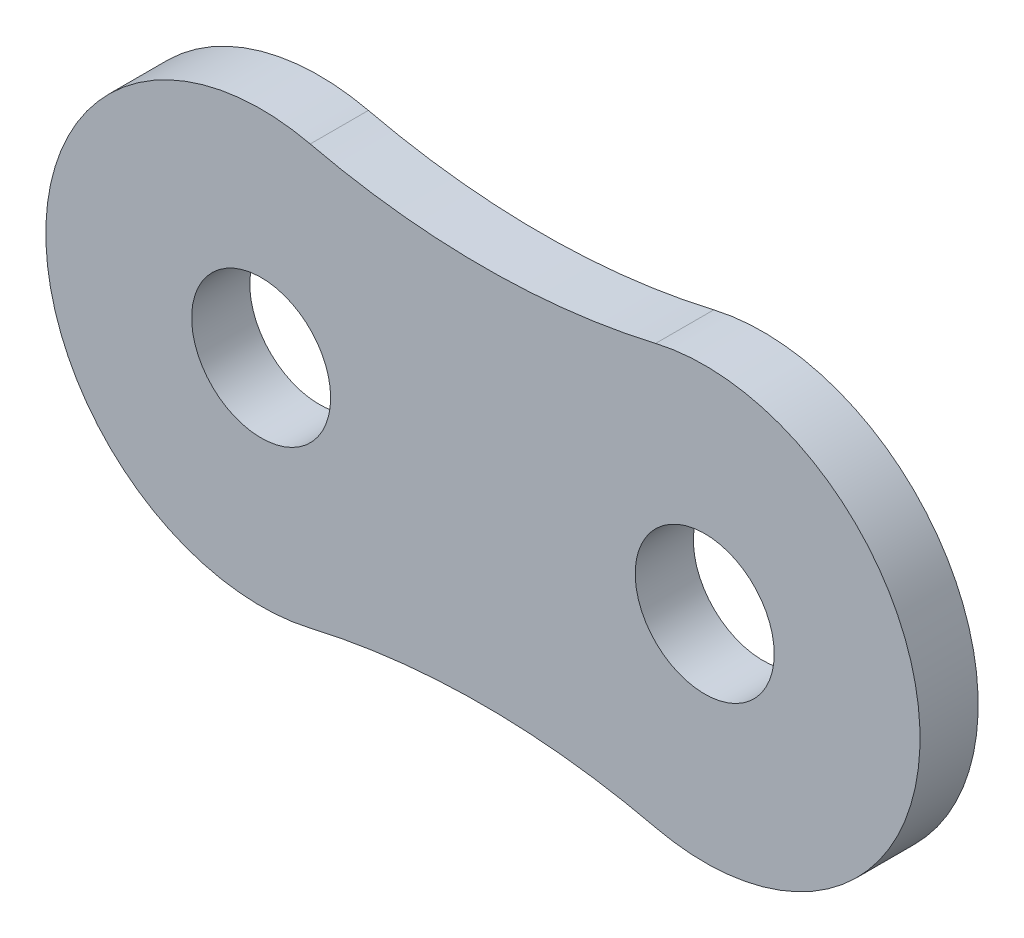
SolidWorks part; units mm, degrees
ref_plane "前视基准面" through (0, 0, 0) normal (0, 0, 1) x (1, 0, 0)
ref_plane "上视基准面" through (0, 0, 0) normal (0, 1, 0) x (1, 0, 0)
ref_plane "右视基准面" through (0, 0, 0) normal (1, 0, 0) x (0, 0, -1)
sketch "草图1" plane through (0, 0, 0) normal (0, 0, 1) x (1, 0, 0)
  line L0 (-6.35, 0) -> (6.35, 0) construction
  line L1 (0, 5.4315) -> (0, -5.4315) construction
  line L2 (6.35, 0) -> (14.2, 0) construction
  line L3 (14.2, 0) -> (25.38, 0) construction
  circle A4 centre (-6.35, 0) radius 6.165
  circle A5 centre (6.35, 0) radius 6.165
  circle A6 centre (0, 27.1196) radius 21.6881
  circle A7 centre (0, -27.1196) radius 21.6881
  circle A8 centre (-6.35, 0) radius 1.99
  circle A9 centre (6.35, 0) radius 1.99
sketch "草图2" plane through (0, 0, 0) normal (0, 0, 1) x (1, 0, 0)
  circle A0 centre (-6.35, 0) radius 6.165 construction
  arc A1 (-4.9445, 6.0026) -> (-4.9445, -6.0026) centre (-6.35, 0) ccw
  circle A2 centre (6.35, 0) radius 6.165 construction
  arc A3 (4.9445, -6.0026) -> (4.9445, 6.0026) centre (6.35, 0) ccw
  circle A4 centre (0, 27.1196) radius 21.6881 construction
  arc A5 (-4.9445, 6.0026) -> (4.9445, 6.0026) centre (0, 27.1196) ccw
  circle A6 centre (0, -27.1196) radius 21.6881 construction
  arc A7 (4.9445, -6.0026) -> (-4.9445, -6.0026) centre (0, -27.1196) ccw
extrude "拉伸1" add sketch "草图2" along normal blind 1.665
sketch "草图3" plane through (0, 0, 1.665) normal (0, 0, 1) x (1, 0, 0)
  circle A0 centre (-6.35, 0) radius 1.99 construction
  circle A1 centre (-6.35, 0) radius 1.99
  circle A2 centre (6.35, 0) radius 1.99 construction
  circle A3 centre (6.35, 0) radius 1.99
extrude "切除-拉伸1" cut sketch "草图3" against normal through all
equation "\"D@拉伸1\" = (  \"b2@草图1\" - \"b1@草图1\" )  / 2"
